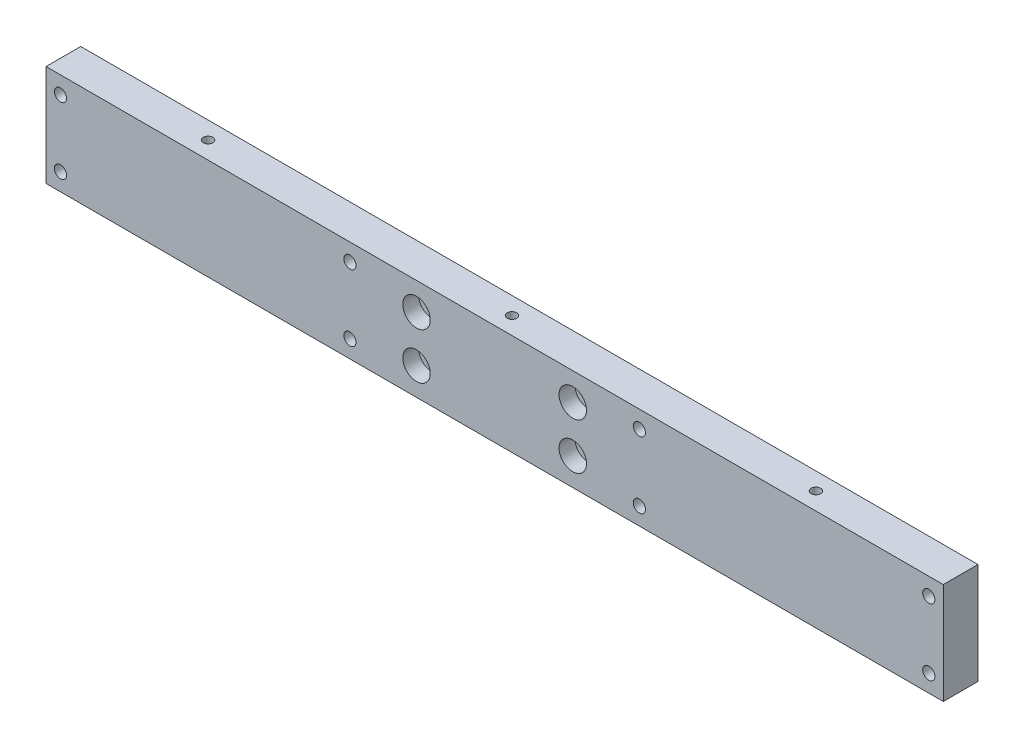
SolidWorks part; units mm, degrees
material "6061 合金"
ref_plane "前基準面" through (0, 0, 0) normal (0, 0, 1) x (1, 0, 0)
ref_plane "上基準面" through (0, 0, 0) normal (0, 1, 0) x (1, 0, 0)
ref_plane "右基準面" through (0, 0, 0) normal (1, 0, 0) x (0, 0, -1)
sketch "草图1" plane through (0, 0, 0) normal (0, 0, 1) x (1, 0, 0)
  line L1 (-155, 17.5) -> (155, 17.5)
  line L2 (-155, 17.5) -> (-155, -17.5)
  line L3 (-155, -17.5) -> (155, -17.5)
  line L4 (155, 17.5) -> (155, -17.5)
  line L5 (-155, 17.5) -> (155, -17.5) construction
  line L6 (-155, -17.5) -> (155, 17.5) construction
  point P0 (0, 0)
  dimension "D1" = 310
  dimension "D2" = 35
extrude "凸台-拉伸1" add sketch "草图1" along normal mid plane 12
hole_wizard "M5 螺纹孔1" positions "草图2" profile "草图3" tap size "M5" standard "ISO" end condition through all
sketch "草图2" plane through (0, 0, 6) normal (0, 0, 1) x (1, 0, 0)
  line L0 (150, 11.5) -> (150, -11.5) construction
  line L2 (150, 0) -> (155, 0) construction
  line L3 (155, -17.5) -> (155, 17.5) construction
  point P0 (150, 11.5)
  point P2 (150, -11.5)
  dimension "D1" = 23
  dimension "D2" = 5
sketch "草图3" plane through (150, 11.5, 6) normal (1, 0, 0) x (0, -1, 0)
  line L0 (0, 0) -> (0, 12)
  line L1 (0, 12) -> (2.1, 12)
  line L2 (2.1, 12) -> (2.1, 0)
  line L5 (2.1, 0) -> (0, 0)
  line L11 (0, -6.35) -> (0, 107.95) construction
  dimension "通孔螺纹孔钻头直径" = 4.2
  dimension "通孔螺纹孔钻头深度" = 12
cosmetic thread "孔螺蚊线1"
cosmetic thread "孔螺蚊线2"
pattern_linear "阵列(线性)2" count 4 spacing 100 along (-1, 0, 0) of "M5 螺纹孔1"
hole_wizard "M5 沉头孔1" positions "草图5" profile "草图4" counterbore size "M5" standard "ISO"
sketch "草图5" plane through (0, 0, 6) normal (0, 0, 1) x (1, 0, 0)
  point P1 (-27, 8)
  point P4 (-27, -8)
  point P7 (27, 8)
  point P10 (27, -8)
sketch "草图4" plane through (-27, 8, 6) normal (1, 0, 0) x (0, -1, 0)
  line L0 (0, 0) -> (0, 12)
  line L1 (0, 12) -> (2.75, 12)
  line L3 (2.75, 12) -> (2.75, 5.5)
  line L4 (2.75, 5.5) -> (4.75, 5.5)
  line L5 (4.75, 5.5) -> (4.75, 0)
  line L7 (4.75, 0) -> (0, 0)
  line L11 (0, -6.35) -> (0, 107.95) construction
  dimension "通孔孔直径" = 5.5
  dimension "通孔孔深度" = 12
  dimension "柱形沉头孔直径" = 9.5
  dimension "柱形沉头孔深度" = 5.5
hole_wizard "M4 螺纹孔1" positions "草图6" profile "草图8" tap size "M4" standard "ISO"
sketch "草图6" plane through (0, 17.5, 0) normal (0, 1, 0) x (1, 0, 0)
  line L0 (105, 0) -> (0, 0) construction
  line L1 (0, 0) -> (-105, 0) construction
  line L3 (-155, -6) -> (-155, 6) construction
  point P1 (105, 0)
  point P3 (0, 0)
  point P6 (-105, 0)
  dimension "D1" = 50
sketch "草图8" plane through (105, 17.5, 0) normal (1, 0, 0) x (0, 0, 1)
  line L0 (0, 0) -> (0, 13.3914)
  line L1 (0, 13.3914) -> (1.65, 12.4)
  line L2 (1.65, 12.4) -> (1.65, 0)
  line L5 (1.65, 0) -> (0, 0)
  line L10 (0, 13.3914) -> (-1.65, 12.4) construction
  line L11 (0, -6.35) -> (0, 107.95) construction
  dimension "螺纹孔钻头直径" = 3.3
  dimension "螺纹孔钻头深度" = 12.4
  dimension "导头角度" = 118
cosmetic thread "孔螺蚊线3" parameters "D1"=8, "D2"=4
cosmetic thread "孔螺蚊线4" parameters "D1"=8, "D2"=4
cosmetic thread "孔螺蚊线5" parameters "D1"=8, "D2"=4
